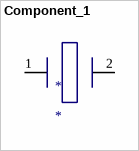
[diagram p0: symbol Component_1]
# Altium schematic symbol library MISC86338-16.SchLib: 1 symbol
Pins are listed as number, name and electrical type; pins without a type are passive.


## Component_1
designator *
footprint XTAL
pins: 1, 2